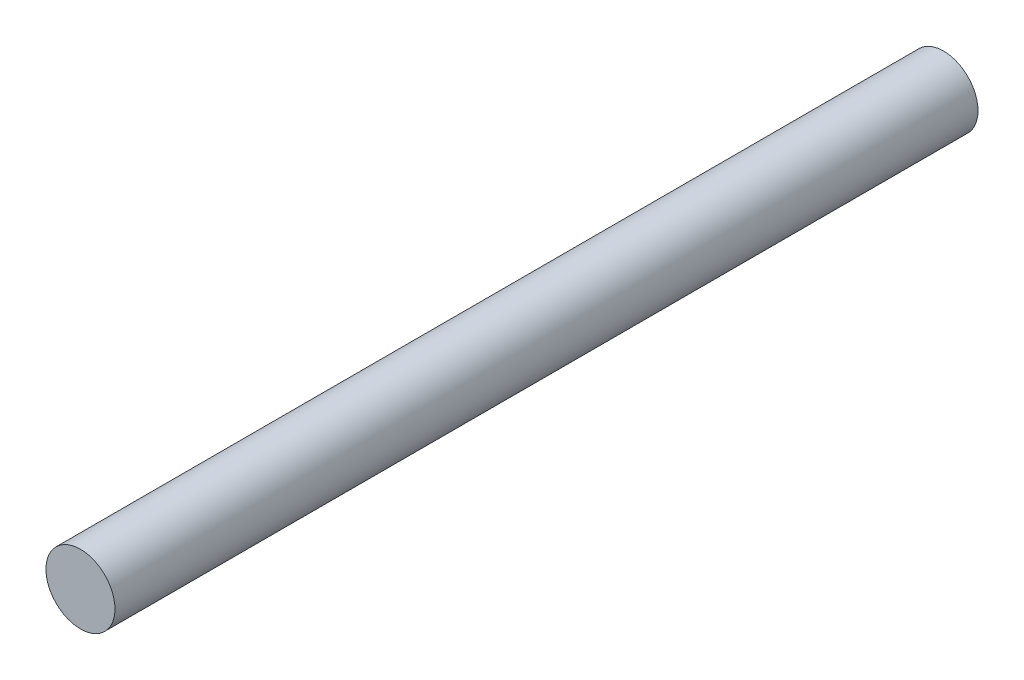
from build123d import *

# Parameters (mm, degrees)
SKETCH1_R           = 20
BOSS_EXTRUDE1_DEPTH = 500


with BuildPart() as part:
    # Sketch1 → Boss-Extrude1 (new body)
    with BuildSketch(Plane.XY):
        Circle(SKETCH1_R)
    extrude(amount=BOSS_EXTRUDE1_DEPTH)


solid = part.part
